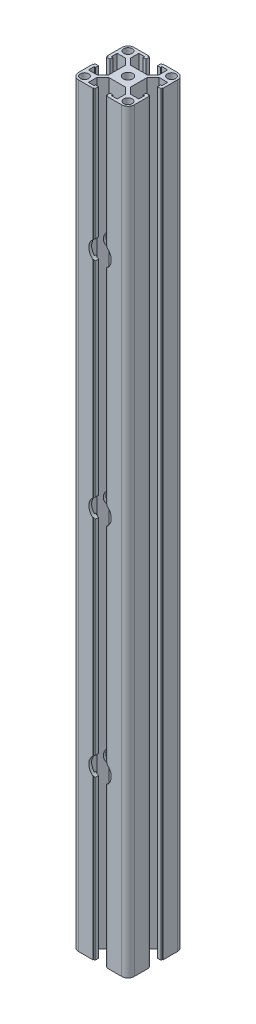
SolidWorks part; units mm, degrees
ref_plane "主视基准图" through (0, 0, 0) normal (0, 0, 1) x (1, 0, 0)
ref_plane "上视基准图" through (0, 0, 0) normal (0, 1, 0) x (1, 0, 0)
ref_plane "右视基准图" through (0, 0, 0) normal (1, 0, 0) x (0, 0, -1)
sketch "草图1" plane through (0, 0, 0) normal (0, 0, 1) x (1, 0, 0)
  line L0 (0, 0) -> (0, 540)
  dimension "D1" = 540
other "结构构件1"
ref_plane "基准面1" through (0, 0, 0) normal (0, 1, 0) x (-1, 0, 0)
sketch "Sketch16" plane through (0, 0, 0) normal (0, 1, 0) x (-1, 0, 0)
  line L0 (-5.1, 20) -> (-5.1, 19.5)
  line L1 (-5.1, 19.5) -> (-4.1, 19.5)
  line L2 (-4.1, 19.5) -> (-4.1, 17)
  line L3 (-6.1, 18) -> (-10.3, 18)
  line L4 (-15.5, -20) -> (-5.1, -20)
  line L5 (-20, -15.5) -> (-20, -5.1)
  line L6 (15.5, 20) -> (5.1, 20)
  line L7 (20, 15.5) -> (20, 5.1)
  line L8 (0, 14.8756) -> (0, 0) construction
  line L9 (0, 0) -> (14.1675, 0) construction
  line L10 (-10.3, 18) -> (-10.3, 12)
  line L11 (-10.3, 12) -> (-6, 7.7)
  line L12 (-6, 7.7) -> (6, 7.7)
  line L13 (10.3, 12) -> (6, 7.7)
  line L14 (10.3, 18) -> (10.3, 12)
  line L15 (6.1, 18) -> (10.3, 18)
  line L16 (4.1, 19.5) -> (4.1, 17)
  line L17 (5.1, 19.5) -> (4.1, 19.5)
  line L18 (5.1, 20) -> (5.1, 19.5)
  line L19 (-5.1, 20) -> (-15.5, 20)
  line L20 (20, 5.1) -> (19.5, 5.1)
  line L21 (0, 0) -> (-15.5563, 15.5563) construction
  line L22 (0, 0) -> (-15.5563, -15.5563) construction
  line L25 (19.5, 5.1) -> (19.5, 4.1)
  line L26 (19.5, 4.1) -> (17, 4.1)
  line L27 (17, 6.1) -> (17, 4.1)
  line L28 (18, 6.1) -> (17, 6.1)
  line L29 (18, 6.1) -> (18, 10.3)
  line L30 (18, 10.3) -> (12, 10.3)
  line L31 (12, 10.3) -> (7.7, 6)
  line L32 (7.7, 6) -> (7.7, -6)
  line L33 (12, -10.3) -> (7.7, -6)
  line L34 (18, -10.3) -> (12, -10.3)
  line L35 (18, -6.1) -> (18, -10.3)
  line L36 (18, -6.1) -> (17, -6.1)
  line L37 (17, -4.1) -> (17, -6.1)
  line L38 (19.5, -4.1) -> (17, -4.1)
  line L39 (19.5, -5.1) -> (19.5, -4.1)
  line L40 (20, -5.1) -> (19.5, -5.1)
  line L41 (5.1, -20) -> (5.1, -19.5)
  line L42 (5.1, -19.5) -> (4.1, -19.5)
  line L43 (4.1, -19.5) -> (4.1, -17)
  line L44 (6.1, -17) -> (4.1, -17)
  line L45 (6.1, -18) -> (6.1, -17)
  line L46 (6.1, -18) -> (10.3, -18)
  line L47 (10.3, -18) -> (10.3, -12)
  line L48 (10.3, -12) -> (6, -7.7)
  line L49 (6, -7.7) -> (-6, -7.7)
  line L50 (-10.3, -12) -> (-6, -7.7)
  line L51 (-10.3, -18) -> (-10.3, -12)
  line L52 (-6.1, -18) -> (-10.3, -18)
  line L53 (-6.1, -18) -> (-6.1, -17)
  line L54 (-4.1, -17) -> (-6.1, -17)
  line L55 (-4.1, -19.5) -> (-4.1, -17)
  line L56 (-5.1, -19.5) -> (-4.1, -19.5)
  line L57 (-5.1, -20) -> (-5.1, -19.5)
  line L58 (-20, -5.1) -> (-19.5, -5.1)
  line L59 (5.1, -20) -> (15.5, -20)
  line L60 (-20, 5.1) -> (-20, 15.5)
  line L61 (-19.5, -5.1) -> (-19.5, -4.1)
  line L62 (-6.1, 18) -> (-6.1, 17)
  line L63 (-6.1, 17) -> (-4.1, 17)
  line L64 (6.1, 18) -> (6.1, 17)
  line L65 (4.1, 17) -> (6.1, 17)
  line L66 (-19.5, -4.1) -> (-17, -4.1)
  line L71 (-17, -6.1) -> (-17, -4.1)
  line L72 (-18, -6.1) -> (-17, -6.1)
  line L73 (-18, -6.1) -> (-18, -10.3)
  line L74 (-18, -10.3) -> (-12, -10.3)
  line L75 (-12, -10.3) -> (-7.7, -6)
  line L76 (-7.7, -6) -> (-7.7, 6)
  line L77 (-12, 10.3) -> (-7.7, 6)
  line L78 (-18, 10.3) -> (-12, 10.3)
  line L79 (-18, 6.1) -> (-18, 10.3)
  line L80 (-18, 6.1) -> (-17, 6.1)
  line L81 (-17, 4.1) -> (-17, 6.1)
  line L82 (-19.5, 4.1) -> (-17, 4.1)
  line L83 (-19.5, 5.1) -> (-19.5, 4.1)
  line L84 (-20, 5.1) -> (-19.5, 5.1)
  line L85 (20, -5.1) -> (20, -15.5)
  circle A0 centre (0, 0) radius 3.4
  arc A1 (-20, 15.5) -> (-15.5, 20) centre (-15.5, 15.5) cw
  arc A2 (20, 15.5) -> (15.5, 20) centre (15.5, 15.5) ccw
  arc A3 (-15.5, -20) -> (-20, -15.5) centre (-15.5, -15.5) cw
  arc A4 (15.5, -20) -> (20, -15.5) centre (15.5, -15.5) ccw
  circle A5 centre (-15.5563, 15.5563) radius 3
  circle A6 centre (15.5563, 15.5563) radius 3
  circle A7 centre (15.5563, -15.5563) radius 3
  circle A8 centre (-15.5563, -15.5563) radius 3
  point P2 (0, 10)
  point P3 (0, 0)
  point P4 (0, 0)
  point P5 (-20, -20)
  point P6 (20, -20)
  point P7 (20, 20)
  point P8 (-20, 20)
  point P36 (-20, 20)
  point P39 (20, 20)
  dimension "D1" = 20.6
  dimension "D2" = 40
  dimension "D3" = 8.2
  dimension "D4" = 10.2
  dimension "D5" = 12.3
  dimension "D6" = 6.8
  dimension "D7" = 4.5
  dimension "D8" = 45
  dimension "D12" = 6
  dimension "D13" = 22
  dimension "D9" = 0.5
  dimension "D10" = 2
  dimension "D11" = 12
  dimension "D16" = 3
  dimension "D17" = 2
hole_wizard "M8 六角凹头螺钉的柱形沉头孔1" positions "草图5" profile "草图4" counterbore size "M8" standard "Iso" end condition through all
sketch "草图5" plane through (9.5819, -44.0931, 20) normal (0, 0, -1) x (-1, 0, 0)
  line L0 (20, 314.0931) -> (-5.9181, 314.0931) construction
  line L2 (-5.9181, 584.0931) -> (-5.9181, 44.0931) construction
  line L6 (9.5819, 44.0931) -> (9.5819, 270.5931) construction
  line L7 (4.4819, 44.0931) -> (-5.9181, 44.0931) construction
  point P0 (9.5819, 164.0931)
  point P2 (9.5819, 324.0931)
  point P26 (9.5819, 484.0931)
  dimension "D1" = 120
  dimension "D2" = 160
  dimension "D3" = 160
sketch "草图4" plane through (0, 120, 20) normal (1, 0, 0) x (0, -1, 0)
  line L0 (0, 0) -> (0, 40)
  line L1 (0, 40) -> (4.5, 40)
  line L3 (4.5, 40) -> (4.5, 12.3)
  line L4 (4.5, 12.3) -> (8, 12.3)
  line L5 (8, 12.3) -> (8, 0)
  line L7 (8, 0) -> (0, 0)
  line L11 (0, -6.35) -> (0, 107.95) construction
  dimension "通孔孔直径" = 9
  dimension "通孔孔深度" = 40
  dimension "柱形沉头孔直径" = 16
  dimension "柱形沉头孔深度" = 12.3
